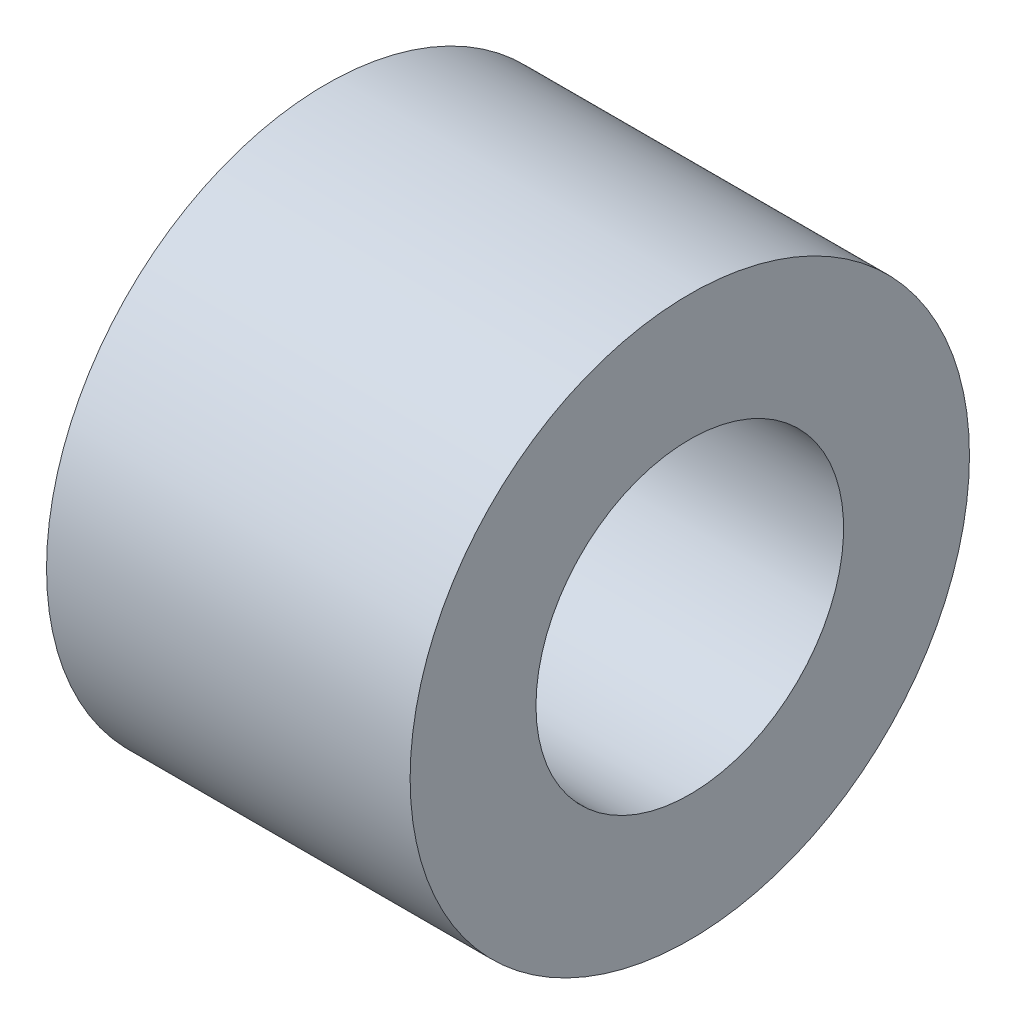
from build123d import *

# Parameters (mm, degrees)
SKETCH2_R           = 10
SKETCH2_R_2         = 5.5
BOSS_EXTRUDE2_DEPTH = 6.5


with BuildPart() as part:
    # Sketch2 → Boss-Extrude2 (new, symmetric)
    with BuildSketch(Plane(origin=(0, 0, 0), x_dir=(0, 0, -1), z_dir=(1, 0, 0))):
        with Locations(Location((0, 0, 0), (0, 0, 180))):
            Circle(SKETCH2_R)
        with Locations(Location((0, 0, 0), (0, 0, 180))):
            Circle(SKETCH2_R_2, mode=Mode.SUBTRACT)
    extrude(amount=BOSS_EXTRUDE2_DEPTH, both=True)


solid = part.part
